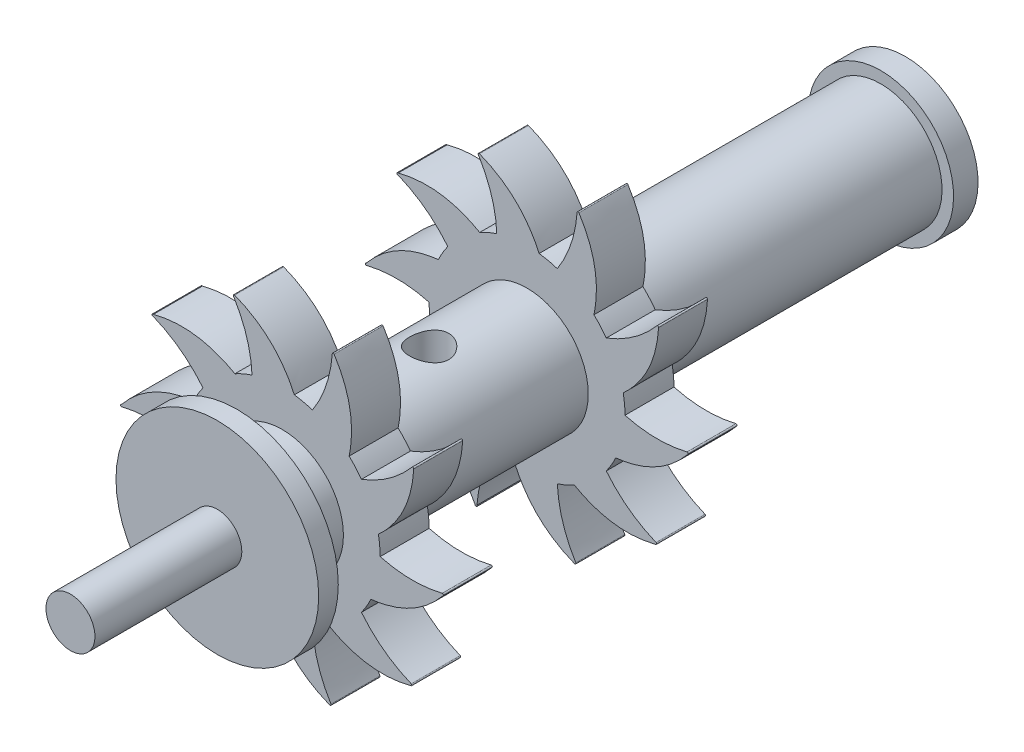
SolidWorks part; units mm, degrees
ref_plane "Front Plane" through (0, 0, 0) normal (0, 0, 1) x (1, 0, 0)
ref_plane "Top Plane" through (0, 0, 0) normal (0, 1, 0) x (1, 0, 0)
ref_plane "Right Plane" through (0, 0, 0) normal (1, 0, 0) x (0, 0, -1)
sketch "Sketch1" plane through (0, 0, 0) normal (0, 0, 1) x (1, 0, 0)
  circle A0 centre (0, 0) radius 12.5
  dimension "D1" = 25
extrude "Boss-Extrude1" add sketch "Sketch1" along normal blind 75
sketch "Sketch2" plane through (0, 0, 2.75) normal (0, 0, -1) x (-1, 0, 0)
  circle A0 centre (0, 0) radius 12.5
  circle A1 centre (0, 0) radius 14.8544
extrude "Boss-Extrude2" add sketch "Sketch2" along normal blind 5
sketch "Sketch3" plane through (0, 0, 75) normal (0, 0, 1) x (1, 0, 0)
  circle A0 centre (0, 0) radius 12.5
extrude "Boss-Extrude3" add sketch "Sketch3" along normal blind 40
sketch "Sketch4" plane through (0, 0, 115) normal (0, 0, 1) x (1, 0, 0)
  line L0 (20, 0) -> (33.2382, 0)
  arc A0 (20, 0) -> (19.6383, 3.7865) centre (0, 0) ccw
  arc A1 (32.8639, -0.4671) -> (32.6623, -0.1459) centre (32.7093, -0.3403) ccw
  arc A2 (26.3129, -19.6948) -> (26.3386, -19.3164) centre (26.2624, -19.5013) ccw
  arc A3 (9.7113, -31.3998) -> (9.9545, -31.1087) centre (9.7841, -31.2135) ccw
  arc A4 (-10.5997, -31.1111) -> (-10.2319, -31.0186) centre (-10.4003, -31.1265) ccw
  arc A5 (-26.862, -18.939) -> (-26.5101, -19.0804) centre (-26.7097, -19.0687) ccw
  arc A6 (-32.8639, 0.4671) -> (-32.6623, 0.1459) centre (-32.8169, 0.2727) ccw
  arc A7 (-26.3129, 19.6948) -> (-26.3386, 19.3164) centre (-26.3892, 19.5099) ccw
  arc A8 (-9.7113, 31.3998) -> (-9.9545, 31.1087) centre (-9.7841, 31.2135) ccw
  arc A9 (10.5997, 31.1111) -> (10.2319, 31.0186) centre (10.4313, 31.0032) ccw
  arc A10 (26.862, 18.939) -> (26.5101, 19.0804) centre (26.6624, 18.9508) ccw
  arc A11 (16.1803, 11.7557) -> (13.662, 14.6065) centre (0, 0) ccw
  arc A12 (6.1803, 19.0211) -> (2.4674, 19.8472) centre (0, 0) ccw
  arc A13 (-6.1803, 19.0211) -> (-9.6698, 17.507) centre (0, 0) ccw
  arc A14 (-16.1803, 11.7557) -> (-18.1134, 8.4797) centre (0, 0) ccw
  arc A15 (-20, 0) -> (-19.6383, -3.7865) centre (0, 0) ccw
  arc A16 (-16.1803, -11.7557) -> (-13.662, -14.6065) centre (0, 0) ccw
  arc A17 (-6.1803, -19.0211) -> (-2.4674, -19.8472) centre (0, 0) ccw
  arc A18 (6.1803, -19.0211) -> (9.6698, -17.507) centre (0, 0) ccw
  arc A19 (16.1803, -11.7557) -> (18.1134, -8.4797) centre (0, 0) ccw
  spline S0 degree 3 poles (32.8639, -0.4671) (29.0265, -5.1458) (24.0849, -7.8294) (18.1134, -8.4797) knots 0.031773 0.031773 0.031773 0.031773 1 1 1 1
  spline S1 degree 3 poles (32.6623, -0.1459) (28.4262, -1.1702) (24.1941, -1.1213) (20, 0) knots 0.04335 0.04335 0.04335 0.04335 1 1 1 1
  spline S2 degree 3 poles (26.3386, -19.3164) (22.3095, -17.6553) (18.9143, -15.1281) (16.1803, -11.7557) knots 0.04335 0.04335 0.04335 0.04335 1 1 1 1
  spline S3 degree 3 poles (26.3129, -19.6948) (20.4583, -21.2244) (14.8831, -20.4909) (9.6698, -17.507) knots 0.031773 0.031773 0.031773 0.031773 1 1 1 1
  spline S4 degree 3 poles (9.9545, -31.1087) (7.6712, -27.3966) (6.41, -23.3564) (6.1803, -19.0211) knots 0.04335 0.04335 0.04335 0.04335 1 1 1 1
  spline S5 degree 3 poles (9.7113, -31.3998) (4.0757, -29.196) (-0.0036, -25.3255) (-2.4674, -19.8472) knots 0.031773 0.031773 0.031773 0.031773 1 1 1 1
  spline S6 degree 3 poles (-10.2319, -31.0186) (-9.8971, -26.6733) (-8.5428, -22.6634) (-6.1803, -19.0211) knots 0.04335 0.04335 0.04335 0.04335 1 1 1 1
  spline S7 degree 3 poles (-10.5997, -31.1111) (-13.8636, -26.0157) (-14.8888, -20.4867) (-13.662, -14.6065) knots 0.031773 0.031773 0.031773 0.031773 1 1 1 1
  spline S8 degree 3 poles (-26.5101, -19.0804) (-23.6851, -15.7618) (-20.2325, -13.3138) (-16.1803, -11.7557) knots 0.04335 0.04335 0.04335 0.04335 1 1 1 1
  spline S9 degree 3 poles (-26.862, -18.939) (-26.5075, -12.8983) (-24.0871, -7.8226) (-19.6383, -3.7865) knots 0.031773 0.031773 0.031773 0.031773 1 1 1 1
  spline S10 degree 3 poles (-32.6623, 0.1459) (-28.4262, 1.1702) (-24.1941, 1.1213) (-20, 0) knots 0.04335 0.04335 0.04335 0.04335 1 1 1 1
  spline S11 degree 3 poles (-32.8639, 0.4671) (-29.0265, 5.1458) (-24.0849, 7.8294) (-18.1134, 8.4797) knots 0.031773 0.031773 0.031773 0.031773 1 1 1 1
  spline S12 degree 3 poles (-26.3386, 19.3164) (-22.3095, 17.6553) (-18.9143, 15.1281) (-16.1803, 11.7557) knots 0.04335 0.04335 0.04335 0.04335 1 1 1 1
  spline S13 degree 3 poles (-26.3129, 19.6948) (-20.4583, 21.2244) (-14.8831, 20.4909) (-9.6698, 17.507) knots 0.031773 0.031773 0.031773 0.031773 1 1 1 1
  spline S14 degree 3 poles (-9.9545, 31.1087) (-7.6712, 27.3966) (-6.3366, 23.3835) (-6.1803, 19.0211) knots 0.04335 0.04335 0.04335 0.04335 1 1 1 1
  spline S15 degree 3 poles (-9.7113, 31.3998) (-4.0757, 29.196) (0.0036, 25.3255) (2.4674, 19.8472) knots 0.031773 0.031773 0.031773 0.031773 1 1 1 1
  spline S16 degree 3 poles (10.2319, 31.0186) (9.8971, 26.6733) (8.5428, 22.6634) (6.1803, 19.0211) knots 0.04335 0.04335 0.04335 0.04335 1 1 1 1
  spline S17 degree 3 poles (10.5997, 31.1111) (13.8636, 26.0157) (14.8888, 20.4867) (13.662, 14.6065) knots 0.031773 0.031773 0.031773 0.031773 1 1 1 1
  spline S18 degree 3 poles (26.5101, 19.0804) (23.6851, 15.7618) (20.2325, 13.3138) (16.1803, 11.7557) knots 0.04335 0.04335 0.04335 0.04335 1 1 1 1
  spline S19 degree 3 poles (26.862, 18.939) (26.5075, 12.8983) (24.0871, 7.8226) (19.6383, 3.7865) knots 0.031773 0.031773 0.031773 0.031773 1 1 1 1
  point P76 (0, 0)
  circle M41 centre (0, 0) radius 12.5
  dimension "D1" = 40
  dimension "D2" = 0.2
extrude "Boss-Extrude4" add sketch "Sketch4" along normal blind 10 contours S19 A10 S18 A11 S17 A9 S16 A12 S15 A8 S14 A13 S13 A7 S12 A14 S11 A6 S10 A15 S9 A5 S8 A16 S7 A4 S6 A17 S5 A3 S4 A18 S3 A2 S2 A19 S0 A1 S1 A0 M41 | M41
sketch "Sketch6" plane through (0, 0, 115) normal (0, 0, -1) x (-1, 0, 0)
  arc A40 (-19.6383, 3.7865) -> (-20, 0) centre (0, 0) ccw
  arc A41 (-32.6623, -0.1459) -> (-32.8639, -0.4671) centre (-32.7093, -0.3403) ccw
  arc A42 (-18.1134, -8.4797) -> (-16.1803, -11.7557) centre (0, 0) ccw
  arc A43 (-26.3386, -19.3164) -> (-26.3129, -19.6948) centre (-26.2624, -19.5013) ccw
  arc A44 (-9.6698, -17.507) -> (-6.1803, -19.0211) centre (0, 0) ccw
  arc A45 (-9.9545, -31.1087) -> (-9.7113, -31.3998) centre (-9.7841, -31.2135) ccw
  arc A46 (2.4674, -19.8472) -> (6.1803, -19.0211) centre (0, 0) ccw
  arc A47 (10.2319, -31.0186) -> (10.5997, -31.1111) centre (10.4003, -31.1265) ccw
  arc A48 (13.662, -14.6065) -> (16.1803, -11.7557) centre (0, 0) ccw
  arc A49 (26.5101, -19.0804) -> (26.862, -18.939) centre (26.7097, -19.0687) ccw
  arc A50 (19.6383, -3.7865) -> (20, 0) centre (0, 0) ccw
  arc A51 (32.6623, 0.1459) -> (32.8639, 0.4671) centre (32.8169, 0.2727) ccw
  arc A52 (18.1134, 8.4797) -> (16.1803, 11.7557) centre (0, 0) ccw
  arc A53 (26.3386, 19.3164) -> (26.3129, 19.6948) centre (26.3892, 19.5099) ccw
  arc A54 (9.6698, 17.507) -> (6.1803, 19.0211) centre (0, 0) ccw
  arc A55 (9.9545, 31.1087) -> (9.7113, 31.3998) centre (9.7841, 31.2135) ccw
  arc A56 (-2.4674, 19.8472) -> (-6.1803, 19.0211) centre (0, 0) ccw
  arc A57 (-10.2319, 31.0186) -> (-10.5997, 31.1111) centre (-10.4313, 31.0032) ccw
  arc A58 (-13.662, 14.6065) -> (-16.1803, 11.7557) centre (0, 0) ccw
  arc A59 (-26.5101, 19.0804) -> (-26.862, 18.939) centre (-26.6624, 18.9508) ccw
  arc A60 (-19.6383, 3.7865) -> (-20, 0) centre (0, 0) ccw
  arc A61 (-32.6623, -0.1459) -> (-32.8639, -0.4671) centre (-32.7093, -0.3403) ccw
  arc A62 (-18.1134, -8.4797) -> (-16.1803, -11.7557) centre (0, 0) ccw
  arc A63 (-26.3386, -19.3164) -> (-26.3129, -19.6948) centre (-26.2624, -19.5013) ccw
  arc A64 (-9.6698, -17.507) -> (-6.1803, -19.0211) centre (0, 0) ccw
  arc A65 (-9.9545, -31.1087) -> (-9.7113, -31.3998) centre (-9.7841, -31.2135) ccw
  arc A66 (2.4674, -19.8472) -> (6.1803, -19.0211) centre (0, 0) ccw
  arc A67 (10.2319, -31.0186) -> (10.5997, -31.1111) centre (10.4003, -31.1265) ccw
  arc A68 (13.662, -14.6065) -> (16.1803, -11.7557) centre (0, 0) ccw
  arc A69 (26.5101, -19.0804) -> (26.862, -18.939) centre (26.7097, -19.0687) ccw
  arc A70 (19.6383, -3.7865) -> (20, 0) centre (0, 0) ccw
  arc A71 (32.6623, 0.1459) -> (32.8639, 0.4671) centre (32.8169, 0.2727) ccw
  arc A72 (18.1134, 8.4797) -> (16.1803, 11.7557) centre (0, 0) ccw
  arc A73 (26.3386, 19.3164) -> (26.3129, 19.6948) centre (26.3892, 19.5099) ccw
  arc A74 (9.6698, 17.507) -> (6.1803, 19.0211) centre (0, 0) ccw
  arc A75 (9.9545, 31.1087) -> (9.7113, 31.3998) centre (9.7841, 31.2135) ccw
  arc A76 (-2.4674, 19.8472) -> (-6.1803, 19.0211) centre (0, 0) ccw
  arc A77 (-10.2319, 31.0186) -> (-10.5997, 31.1111) centre (-10.4313, 31.0032) ccw
  arc A78 (-13.662, 14.6065) -> (-16.1803, 11.7557) centre (0, 0) ccw
  arc A79 (-26.5101, 19.0804) -> (-26.862, 18.939) centre (-26.6624, 18.9508) ccw
  spline S40 degree 3 poles (2795.2302, 953.3649) (-1294.926, 346.2764) (-516.9976, -1192.5688) (2444.6267, 1665.6283) knots -19.544212 -19.544212 -19.544212 -19.544212 20.652733 20.652733 20.652733 20.652733 only from (-26.862, 18.939) to (-19.6383, 3.7865)
  spline S41 degree 3 poles (-636.6604, 2896.2319) (1051.8157, -939.2729) (-1061.9342, -1001.8006) (461.7845, 2920.0992) knots -28.28974 -28.28974 -28.28974 -28.28974 29.233184 29.233184 29.233184 29.233184 only from (-20, 0) to (-32.6623, -0.1459)
  spline S42 degree 3 poles (1701.0149, 2414.2835) (-1251.1533, -480.9949) (282.7145, -1268.692) (998.7128, 2784.4371) knots -19.544212 -19.544212 -19.544212 -19.544212 20.652733 20.652733 20.652733 20.652733 only from (-32.8639, -0.4671) to (-18.1134, -8.4797)
  spline S43 degree 3 poles (-2217.4315, 1968.8813) (1403.0275, -141.646) (-270.2792, -1434.663) (-1342.7997, 2633.84) knots -28.28974 -28.28974 -28.28974 -28.28974 29.233184 29.233184 29.233184 29.233184 only from (-16.1803, -11.7557) to (-26.3386, -19.3164)
  spline S44 degree 3 poles (-42.9302, 2953.0279) (-729.4826, -1124.5425) (974.4393, -860.2179) (-828.6755, 2839.6856) knots -19.544212 -19.544212 -19.544212 -19.544212 20.652733 20.652733 20.652733 20.652733 only from (-26.3129, -19.6948) to (-9.6698, -17.507)
  spline S45 degree 3 poles (-2951.2191, 289.4849) (1218.3305, 710.0849) (624.6133, -1319.5329) (-2634.4801, 1341.5434) knots -28.28974 -28.28974 -28.28974 -28.28974 29.233184 29.233184 29.233184 29.233184 only from (-6.1803, -19.0211) to (-9.9545, -31.1087)
  spline S46 degree 3 poles (-1770.4775, 2363.816) (70.8257, -1338.5531) (1293.9613, -123.1699) (-2339.5379, 1810.2707) knots -19.544212 -19.544212 -19.544212 -19.544212 20.652733 20.652733 20.652733 20.652733 only from (-9.7113, -31.3998) to (2.4674, -19.8472)
  spline S47 degree 3 poles (-2557.7414, -1500.4849) (568.2726, 1290.5874) (1280.9247, -700.3861) (-2919.8786, -463.1771) knots -28.28974 -28.28974 -28.28974 -28.28974 29.233184 29.233184 29.233184 29.233184 only from (6.1803, -19.0211) to (10.2319, -31.0186)
  spline S48 degree 3 poles (-2821.7626, 871.7067) (844.081, -1041.2819) (1119.2342, 660.9249) (-2956.7763, 89.3939) knots -19.544212 -19.544212 -19.544212 -19.544212 20.652733 20.652733 20.652733 20.652733 only from (10.5997, -31.1111) to (13.662, -14.6065)
  spline S49 degree 3 poles (-1187.2933, -2717.3204) (-298.846, 1378.1294) (1447.9665, 186.2844) (-2089.9827, -2090.9798) knots -28.28974 -28.28974 -28.28974 -28.28974 29.233184 29.233184 29.233184 29.233184 only from (16.1803, -11.7557) to (26.5101, -19.0804)
  spline S50 degree 3 poles (-2795.2302, -953.3649) (1294.926, -346.2764) (516.9976, 1192.5688) (-2444.6267, -1665.6283) knots -19.544212 -19.544212 -19.544212 -19.544212 20.652733 20.652733 20.652733 20.652733 only from (26.862, -18.939) to (19.6383, -3.7865)
  spline S51 degree 3 poles (636.6604, -2896.2319) (-1051.8157, 939.2729) (1061.9342, 1001.8006) (-461.7845, -2920.0992) knots -28.28974 -28.28974 -28.28974 -28.28974 29.233184 29.233184 29.233184 29.233184 only from (20, 0) to (32.6623, 0.1459)
  spline S52 degree 3 poles (-1701.0149, -2414.2835) (1251.1533, 480.9949) (-282.7145, 1268.692) (-998.7128, -2784.4371) knots -19.544212 -19.544212 -19.544212 -19.544212 20.652733 20.652733 20.652733 20.652733 only from (32.8639, 0.4671) to (18.1134, 8.4797)
  spline S53 degree 3 poles (2217.4315, -1968.8813) (-1403.0275, 141.646) (270.2792, 1434.663) (1342.7997, -2633.84) knots -28.28974 -28.28974 -28.28974 -28.28974 29.233184 29.233184 29.233184 29.233184 only from (16.1803, 11.7557) to (26.3386, 19.3164)
  spline S54 degree 3 poles (42.9302, -2953.0279) (729.4826, 1124.5425) (-974.4393, 860.2179) (828.6755, -2839.6856) knots -19.544212 -19.544212 -19.544212 -19.544212 20.652733 20.652733 20.652733 20.652733 only from (26.3129, 19.6948) to (9.6698, 17.507)
  spline S55 degree 3 poles (2843.3633, -939.2765) (-3363.1572, 771.7566) (3580.6882, -533.3656) (-2894.274, 757.1505) knots -18.120369 -18.120369 -18.120369 -18.120369 28.495583 28.495583 28.495583 28.495583 only from (6.1803, 19.0211) to (9.9545, 31.1087)
  spline S56 degree 3 poles (1770.4775, -2363.816) (-70.8257, 1338.5531) (-1293.9613, 123.1699) (2339.5379, -1810.2707) knots -19.544212 -19.544212 -19.544212 -19.544212 20.652733 20.652733 20.652733 20.652733 only from (9.7113, 31.3998) to (-2.4674, 19.8472)
  spline S57 degree 3 poles (2557.7414, 1500.4849) (-568.2726, -1290.5874) (-1280.9247, 700.3861) (2919.8786, 463.1771) knots -28.28974 -28.28974 -28.28974 -28.28974 29.233184 29.233184 29.233184 29.233184 only from (-6.1803, 19.0211) to (-10.2319, 31.0186)
  spline S58 degree 3 poles (2821.7626, -871.7067) (-844.081, 1041.2819) (-1119.2342, -660.9249) (2956.7763, -89.3939) knots -19.544212 -19.544212 -19.544212 -19.544212 20.652733 20.652733 20.652733 20.652733 only from (-10.5997, 31.1111) to (-13.662, 14.6065)
  spline S59 degree 3 poles (1187.2933, 2717.3204) (298.846, -1378.1294) (-1447.9665, -186.2844) (2089.9827, 2090.9798) knots -28.28974 -28.28974 -28.28974 -28.28974 29.233184 29.233184 29.233184 29.233184 only from (-16.1803, 11.7557) to (-26.5101, 19.0804)
  spline S60 degree 3 poles (-26.862, 18.939) (-26.5075, 12.8983) (-24.0871, 7.8226) (-19.6383, 3.7865) knots 0.031773 0.031773 0.031773 0.031773 1 1 1 1
  spline S61 degree 3 poles (-20, 0) (-24.1941, -1.1213) (-28.4262, -1.1702) (-32.6623, -0.1459) knots 0.04335 0.04335 0.04335 0.04335 1 1 1 1
  spline S62 degree 3 poles (-32.8639, -0.4671) (-29.0265, -5.1458) (-24.0849, -7.8294) (-18.1134, -8.4797) knots 0.031773 0.031773 0.031773 0.031773 1 1 1 1
  spline S63 degree 3 poles (-16.1803, -11.7557) (-18.9143, -15.1281) (-22.3095, -17.6553) (-26.3386, -19.3164) knots 0.04335 0.04335 0.04335 0.04335 1 1 1 1
  spline S64 degree 3 poles (-26.3129, -19.6948) (-20.4583, -21.2244) (-14.8831, -20.4909) (-9.6698, -17.507) knots 0.031773 0.031773 0.031773 0.031773 1 1 1 1
  spline S65 degree 3 poles (-6.1803, -19.0211) (-6.41, -23.3564) (-7.6712, -27.3966) (-9.9545, -31.1087) knots 0.04335 0.04335 0.04335 0.04335 1 1 1 1
  spline S66 degree 3 poles (-9.7113, -31.3998) (-4.0757, -29.196) (0.0036, -25.3255) (2.4674, -19.8472) knots 0.031773 0.031773 0.031773 0.031773 1 1 1 1
  spline S67 degree 3 poles (6.1803, -19.0211) (8.5428, -22.6634) (9.8971, -26.6733) (10.2319, -31.0186) knots 0.04335 0.04335 0.04335 0.04335 1 1 1 1
  spline S68 degree 3 poles (10.5997, -31.1111) (13.8636, -26.0157) (14.8888, -20.4867) (13.662, -14.6065) knots 0.031773 0.031773 0.031773 0.031773 1 1 1 1
  spline S69 degree 3 poles (16.1803, -11.7557) (20.2325, -13.3138) (23.6851, -15.7618) (26.5101, -19.0804) knots 0.04335 0.04335 0.04335 0.04335 1 1 1 1
  spline S70 degree 3 poles (26.862, -18.939) (26.5075, -12.8983) (24.0871, -7.8226) (19.6383, -3.7865) knots 0.031773 0.031773 0.031773 0.031773 1 1 1 1
  spline S71 degree 3 poles (20, 0) (24.1941, 1.1213) (28.4262, 1.1702) (32.6623, 0.1459) knots 0.04335 0.04335 0.04335 0.04335 1 1 1 1
  spline S72 degree 3 poles (32.8639, 0.4671) (29.0265, 5.1458) (24.0849, 7.8294) (18.1134, 8.4797) knots 0.031773 0.031773 0.031773 0.031773 1 1 1 1
  spline S73 degree 3 poles (16.1803, 11.7557) (18.9143, 15.1281) (22.3095, 17.6553) (26.3386, 19.3164) knots 0.04335 0.04335 0.04335 0.04335 1 1 1 1
  spline S74 degree 3 poles (26.3129, 19.6948) (20.4583, 21.2244) (14.8831, 20.4909) (9.6698, 17.507) knots 0.031773 0.031773 0.031773 0.031773 1 1 1 1
  spline S75 degree 3 poles (6.1803, 19.0211) (6.3366, 23.3835) (7.6712, 27.3966) (9.9545, 31.1087) knots 0.04335 0.04335 0.04335 0.04335 1 1 1 1
  spline S76 degree 3 poles (9.7113, 31.3998) (4.0757, 29.196) (-0.0036, 25.3255) (-2.4674, 19.8472) knots 0.031773 0.031773 0.031773 0.031773 1 1 1 1
  spline S77 degree 3 poles (-6.1803, 19.0211) (-8.5428, 22.6634) (-9.8971, 26.6733) (-10.2319, 31.0186) knots 0.04335 0.04335 0.04335 0.04335 1 1 1 1
  spline S78 degree 3 poles (-10.5997, 31.1111) (-13.8636, 26.0157) (-14.8888, 20.4867) (-13.662, 14.6065) knots 0.031773 0.031773 0.031773 0.031773 1 1 1 1
  spline S79 degree 3 poles (-16.1803, 11.7557) (-20.2325, 13.3138) (-23.6851, 15.7618) (-26.5101, 19.0804) knots 0.04335 0.04335 0.04335 0.04335 1 1 1 1
  dimension "D1" = 0
extrude "Boss-Extrude5" add sketch "Sketch6" along normal blind 8 from offset 40
sketch "Sketch5" plane through (0, 0, 0) normal (0, 1, 0) x (1, 0, 0)
  line L0 (-12.5, -75) -> (12.5, -75) construction
  line L1 (2.4674, -115) -> (-9.7113, -115) construction
  circle A0 centre (0, -95) radius 4
  dimension "D1" = 8
  dimension "D2" = 40
  dimension "D3" = 20
extrude "Cut-Extrude1" cut sketch "Sketch5" against normal blind 34 and the other way blind 41
ref_plane "Plane1" through (0, 0, 95) normal (0, 0, -1) x (-1, 0, 0)
mirror "Mirror1" about plane through (0, 0, 95) normal (0, 0, -1) of bodies 110
sketch "Sketch7" plane through (0, 0, 192.25) normal (0, 0, 1) x (1, 0, 0)
  circle A0 centre (0, 0) radius 15.3333
extrude "Cut-Extrude2" cut sketch "Sketch7" against normal blind 58
sketch "Sketch8" plane through (0, 0, 134.25) normal (0, 0, 1) x (1, 0, 0)
  circle A0 centre (0, 0) radius 20.7
  dimension "D1" = 41.4
extrude "Boss-Extrude6" add sketch "Sketch8" along normal blind 4
sketch "Sketch9" plane through (0, 0, 138.25) normal (0, 0, 1) x (1, 0, 0)
  circle A0 centre (0, 0) radius 5
  dimension "D1" = 10
extrude "Boss-Extrude7" add sketch "Sketch9" along normal blind 30
